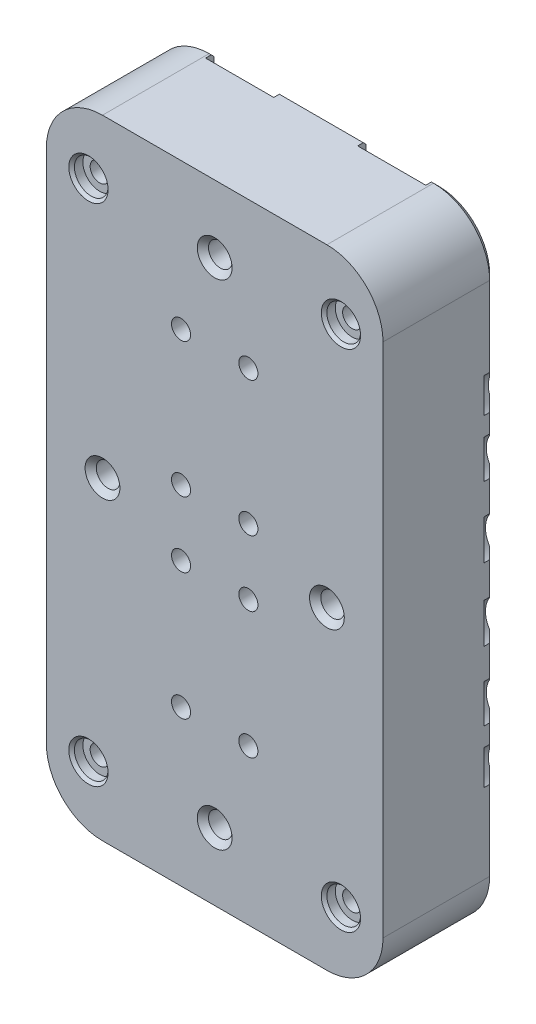
from build123d import *

# Parameters (mm, degrees)
EXTRUDE_1_DEPTH             = 20
HOLE_WIZARD_M4_1_D          = 3.3
SKETCH_4_R                  = 3
CUT_EXTRUDE_1_DEPTH         = 2
HOLE_WIZARD_0_D             = 3.4
HOLE_WIZARD_0_CBORE_D       = 6
HOLE_WIZARD_0_CBORE_DEPTH   = 4
HOLE_WIZARD_0_2_D           = 3.4
HOLE_WIZARD_0_2_CBORE_D     = 6
HOLE_WIZARD_0_2_CBORE_DEPTH = 4
HOLE_WIZARD_2_D             = 3.4
HOLE_WIZARD_2_CBORE_D       = 6
HOLE_WIZARD_2_CBORE_DEPTH   = 4
SKETCH_15_R                 = 6.5
CUT_EXTRUDE_3_DEPTH         = 8.5
SKETCH_16_R                 = 6.5
CUT_EXTRUDE_4_DEPTH         = 8.5
HOLE_WIZARD_M4_2_D          = 3.3
HOLE_WIZARD_M5_2_D          = 4.2
HOLE_WIZARD_M5_2_DEPTH      = 7
HOLE_WIZARD_M5_2_TIP        = 1.2618073
CHAMFER_1_SIZE              = 1
CUT_EXTRUDE_5_DEPTH         = 2
SKETCH_24_W                 = 12.147413759
SKETCH_24_H                 = 6.271213277
CUT_EXTRUDE_6_DEPTH         = 2
SKETCH_25_R                 = 4.5
CUT_EXTRUDE_7_DEPTH         = 2
FILLET_1_R                  = 2
CHAMFER_2_SIZE              = 0.5
CHAMFER_3_SIZE              = 0.5
CHAMFER_4_SIZE              = 1


with BuildPart() as part:
    # 草图1 → 凸台-拉伸1 (new body)
    with BuildSketch(Plane.XY):
        with BuildLine():
            Line((-30, 46), (-30, -46))
            ThreePointArc((-30, -46), (-27.071067812, -53.071067812), (-20, -56))
            Line((-20, -56), (20, -56))
            ThreePointArc((20, -56), (27.071067812, -53.071067812), (30, -46))
            Line((30, -46), (30, 46))
            ThreePointArc((30, 46), (27.071067812, 53.071067812), (20, 56))
            Line((20, 56), (-20, 56))
            ThreePointArc((-20, 56), (-27.071067812, 53.071067812), (-30, 46))
        make_face()
    extrude(amount=EXTRUDE_1_DEPTH)

    # M4 螺纹孔1 (through all)
    with Locations(Plane.XY.offset(20)):
        with Locations((22.5, -45), (-22.5, -45), (-22.5, 45), (22.5, 45), (-112.393620691, 267.430767935)):
            Hole(HOLE_WIZARD_M4_1_D / 2)

    # 草图4 → 切除-拉伸1 (cut)
    with BuildSketch(Plane.XY.offset(20)):
        with Locations((22.5, -45)):
            Circle(SKETCH_4_R)
        with Locations((-22.5, -45)):
            Circle(SKETCH_4_R)
        with Locations((22.5, 45)):
            Circle(SKETCH_4_R)
        with Locations((-22.5, 45)):
            Circle(SKETCH_4_R)
    extrude(amount=-CUT_EXTRUDE_1_DEPTH, mode=Mode.SUBTRACT)

    # Hole Wizard 0 (through all)
    with Locations(Plane(origin=(0, 0, 0), x_dir=(-1, 0, 0), z_dir=(0, 0, -1))):
        with Locations((22.5, 45), (-22.5, -45), (-22.5, 45), (22.5, -45)):
            CounterBoreHole(HOLE_WIZARD_0_D / 2, HOLE_WIZARD_0_CBORE_D / 2, HOLE_WIZARD_0_CBORE_DEPTH)

    # Hole Wizard 0 2 (through all)
    with Locations(Plane(origin=(0, 0, 0), x_dir=(-1, 0, 0), z_dir=(0, 0, -1))):
        with Locations((6, 5.95), (-6, 5.95), (6, 29.95), (-6, 29.95)):
            CounterBoreHole(HOLE_WIZARD_0_2_D / 2, HOLE_WIZARD_0_2_CBORE_D / 2, HOLE_WIZARD_0_2_CBORE_DEPTH)

    # 大小六角凹头盖螺钉柱孔2 (through all)
    with Locations(Plane(origin=(0, 0, 0), x_dir=(-1, 0, 0), z_dir=(0, 0, -1))):
        with Locations((-6, -5.75), (6, -5.75), (-6, -28.35), (6, -28.35)):
            CounterBoreHole(HOLE_WIZARD_2_D / 2, HOLE_WIZARD_2_CBORE_D / 2, HOLE_WIZARD_2_CBORE_DEPTH)

    # 草图15 → 切除-拉伸3 (cut)
    with BuildSketch(Plane.XY):
        with Locations((0, -44)):
            Circle(SKETCH_15_R)
        with Locations((0, 44)):
            Circle(SKETCH_15_R)
    extrude(amount=CUT_EXTRUDE_3_DEPTH, mode=Mode.SUBTRACT)

    # 草图16 → 切除-拉伸4 (cut)
    with BuildSketch(Plane(origin=(0, 0, 0), x_dir=(-1, 0, 0), z_dir=(0, 0, -1))):
        with Locations((-20, -0.000113892)):
            Circle(SKETCH_16_R)
        with Locations((20, -0.000113892)):
            Circle(SKETCH_16_R)
    extrude(amount=-CUT_EXTRUDE_4_DEPTH, mode=Mode.SUBTRACT)

    # M4 螺纹孔2 (through all)
    with Locations(Plane(origin=(0, 0, 8.5), x_dir=(-1, 0, 0), z_dir=(0, 0, -1))):
        with Locations((-20, -0.000113892), (20, -0.000113892), (0, 44), (0, -44)):
            Hole(HOLE_WIZARD_M4_2_D / 2)

    # M5 螺纹孔2
    with Locations(Plane.XY.offset(20)):
        with Locations((20, -0.000113892), (-20, -0.000113892), (0, 44), (0, -44)):
            Hole(HOLE_WIZARD_M5_2_D / 2, depth=HOLE_WIZARD_M5_2_DEPTH)
            with Locations((0, 0, -(HOLE_WIZARD_M5_2_DEPTH + HOLE_WIZARD_M5_2_TIP / 2))):  # 118° drill point
                Cone(0, HOLE_WIZARD_M5_2_D / 2, HOLE_WIZARD_M5_2_TIP, mode=Mode.SUBTRACT)

    # 倒角1
    chamfer_1_edges = [part.edges().sort_by_distance(p)[0] for p in [
        (0, -56, 0),
        (-27.071067812, -53.071067812, 0),
        (-30, 0, 0),
        (-27.071067812, 53.071067812, 0),
        (0, 56, 0),
        (27.071067812, 53.071067812, 0),
        (30, 0, 0),
        (27.071067812, -53.071067812, 0),
    ]]
    chamfer(chamfer_1_edges, length=CHAMFER_1_SIZE)

    # 草图23 → 切除-拉伸5 (cut)
    with BuildSketch(Plane(origin=(0, 0, 0), x_dir=(-1, 0, 0), z_dir=(0, 0, -1))):
        with BuildLine():
            ThreePointArc((-22.323817271, -27.335113738), (-17.462363329, -33.173780323), (-14.245473517, -26.290802635))
            ThreePointArc((-14.245473517, -26.290802635), (-19.106927458, -20.45213605), (-22.323817271, -27.335113738))
        make_face()
        with BuildLine():
            ThreePointArc((14.245473517, -26.290802635), (19.106927458, -20.45213605), (22.323817271, -27.335113738))
            ThreePointArc((22.323817271, -27.335113738), (17.462363329, -33.173780323), (14.245473517, -26.290802635))
        make_face()
        with BuildLine():
            ThreePointArc((22.323817271, 27.335113738), (17.462363329, 33.173780323), (14.245473517, 26.290802635))
            ThreePointArc((14.245473517, 26.290802635), (19.106927458, 20.45213605), (22.323817271, 27.335113738))
        make_face()
        with BuildLine():
            ThreePointArc((-14.245473517, 26.290802635), (-19.106927458, 20.45213605), (-22.323817271, 27.335113738))
            ThreePointArc((-22.323817271, 27.335113738), (-17.462363329, 33.173780323), (-14.245473517, 26.290802635))
        make_face()
    extrude(amount=-CUT_EXTRUDE_5_DEPTH, mode=Mode.SUBTRACT)

    # 草图24 → 切除-拉伸6 (cut)
    with BuildSketch(Plane(origin=(0, 0, 0), x_dir=(-1, 0, 0), z_dir=(0, 0, -1))):
        with Locations((-13.55276297, -52.864393362)):
            Rectangle(SKETCH_24_W, SKETCH_24_H)
        with Locations((-13.55276297, 52.864393362)):
            Rectangle(SKETCH_24_W, SKETCH_24_H)
        with Locations((13.55276297, 52.864393362)):
            Rectangle(SKETCH_24_W, SKETCH_24_H)
        with Locations((13.55276297, -52.864393362)):
            Rectangle(SKETCH_24_W, SKETCH_24_H)
    extrude(amount=-CUT_EXTRUDE_6_DEPTH, mode=Mode.SUBTRACT)

    # 草图25 → 切除-拉伸7 (cut)
    with BuildSketch(Plane(origin=(0, 0, 0), x_dir=(-1, 0, 0), z_dir=(0, 0, -1))):
        with Locations((-32.759999968, 6.439999977)):
            Circle(SKETCH_25_R)
        with Locations((-32.910000001, -18.864999981)):
            Circle(SKETCH_25_R)
        with Locations((-33.274795201, -28.710916372)):
            Circle(SKETCH_25_R)
        with Locations((33.274795201, -28.710916372)):
            Circle(SKETCH_25_R)
        with Locations((32.910000001, -18.864999981)):
            Circle(SKETCH_25_R)
        with Locations((32.759999968, 6.439999977)):
            Circle(SKETCH_25_R)
        with Locations((32.759999968, -6.439999977)):
            Circle(SKETCH_25_R)
        with Locations((32.910000001, 18.864999981)):
            Circle(SKETCH_25_R)
        with Locations((33.274795201, 28.710916372)):
            Circle(SKETCH_25_R)
        with Locations((-33.274795201, 28.710916372)):
            Circle(SKETCH_25_R)
        with Locations((-32.910000001, 18.864999981)):
            Circle(SKETCH_25_R)
        with Locations((-32.759999968, -6.439999977)):
            Circle(SKETCH_25_R)
    extrude(amount=-CUT_EXTRUDE_7_DEPTH, mode=Mode.SUBTRACT)

    # 圆角1
    fillet_1_edges = [part.edges().sort_by_distance(p)[0] for p in [
        (7.47905609, -49.728786723, 1),
        (19.626469849, -49.728786723, 1),
        (7.47905609, 49.728786723, 1),
        (19.626469849, 49.728786723, 1),
        (-7.47905609, 49.728786723, 1),
        (-19.626469849, 49.728786723, 1),
        (-7.47905609, -49.728786723, 1),
        (-19.626469849, -49.728786723, 1),
    ]]
    fillet(fillet_1_edges, radius=FILLET_1_R)

    # 倒角2
    chamfer_2_edges = [part.edges().sort_by_distance(p)[0] for p in [
        (9, 29.95, 0),
        (-3, 29.95, 0),
        (9, 5.95, 0),
        (-3, 5.95, 0),
        (-3, -28.35, 0),
        (9, -28.35, 0),
        (-3, -5.75, 0),
        (9, -5.75, 0),
        (-6.5, -44, 0),
        (26.5, -0.000113892, 0),
        (-13.5, -0.000113892, 0),
        (19.106927458, -20.45213605, 0),
        (17.462363329, -33.173780323, 0),
        (-17.462363329, -33.173780323, 0),
        (-19.106927458, -20.45213605, 0),
        (-19.106927458, 20.45213605, 0),
        (-17.462363329, 33.173780323, 0),
        (17.462363329, 33.173780323, 0),
        (19.106927458, 20.45213605, 0),
        (7.47905609, -53.364393362, 0),
        (19.626469849, 53.364393362, 0),
        (-7.47905609, 53.364393362, 0),
        (-19.626469849, -53.364393362, 0),
        (13.552762969, 49.728786723, 0),
        (7.47905609, 53.364393362, 0),
        (-19.626469849, 53.364393362, 0),
        (-13.552762969, 49.728786723, 0),
        (-7.47905609, -53.364393362, 0),
        (-13.552762969, -49.728786723, 0),
        (13.552762969, -49.728786723, 0),
        (19.626469849, -53.364393362, 0),
        (19.040683411, 50.314573161, 0),
        (8.064842527, 50.314573161, 0),
        (-19.040683411, 50.314573161, 0),
        (-8.064842527, 50.314573161, 0),
        (-8.064842527, -50.314573161, 0),
        (-19.040683411, -50.314573161, 0),
        (8.064842527, -50.314573161, 0),
        (19.040683411, -50.314573161, 0),
        (-19.5, -45, 0),
        (25.5, 45, 0),
        (25.5, 45, 4),
        (25.5, -45, 0),
        (-19.5, 45, 0),
    ]]
    chamfer(chamfer_2_edges, length=CHAMFER_2_SIZE)

    # 倒角3
    chamfer_3_edges = [part.edges().sort_by_distance(p)[0] for p in [
        (19.5, -45, 20),
        (-25.5, -45, 20),
        (19.5, 45, 20),
        (-25.5, 45, 20),
    ]]
    chamfer(chamfer_3_edges, length=CHAMFER_3_SIZE)

    # 倒角4
    chamfer_4_edges = [part.edges().sort_by_distance(p)[0] for p in [
        (2.1, -44, 20),
        (2.1, 44, 20),
        (-17.9, -0.000113892, 20),
        (22.1, -0.000113892, 20),
    ]]
    chamfer(chamfer_4_edges, length=CHAMFER_4_SIZE)


solid = part.part
